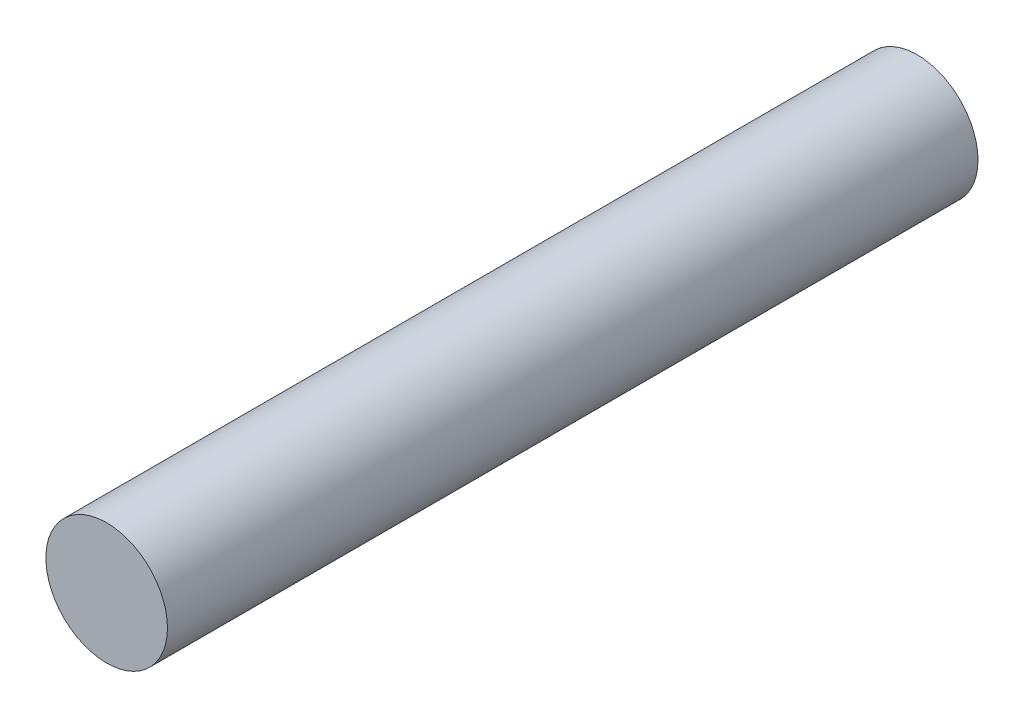
SolidWorks part; units mm, degrees
material "Buche"
ref_plane "Front Plane" through (0, 0, 0) normal (0, 0, 1) x (1, 0, 0)
ref_plane "Top Plane" through (0, 0, 0) normal (0, 1, 0) x (1, 0, 0)
ref_plane "Right Plane" through (0, 0, 0) normal (1, 0, 0) x (0, 0, -1)
sketch "Sketch1" plane through (0, 0, 0) normal (0, 0, 1) x (1, 0, 0)
  circle A0 centre (0, 0) radius 75
  dimension "Durchmesser" = 150
extrude "Length" add sketch "Sketch1" along normal blind 1000
